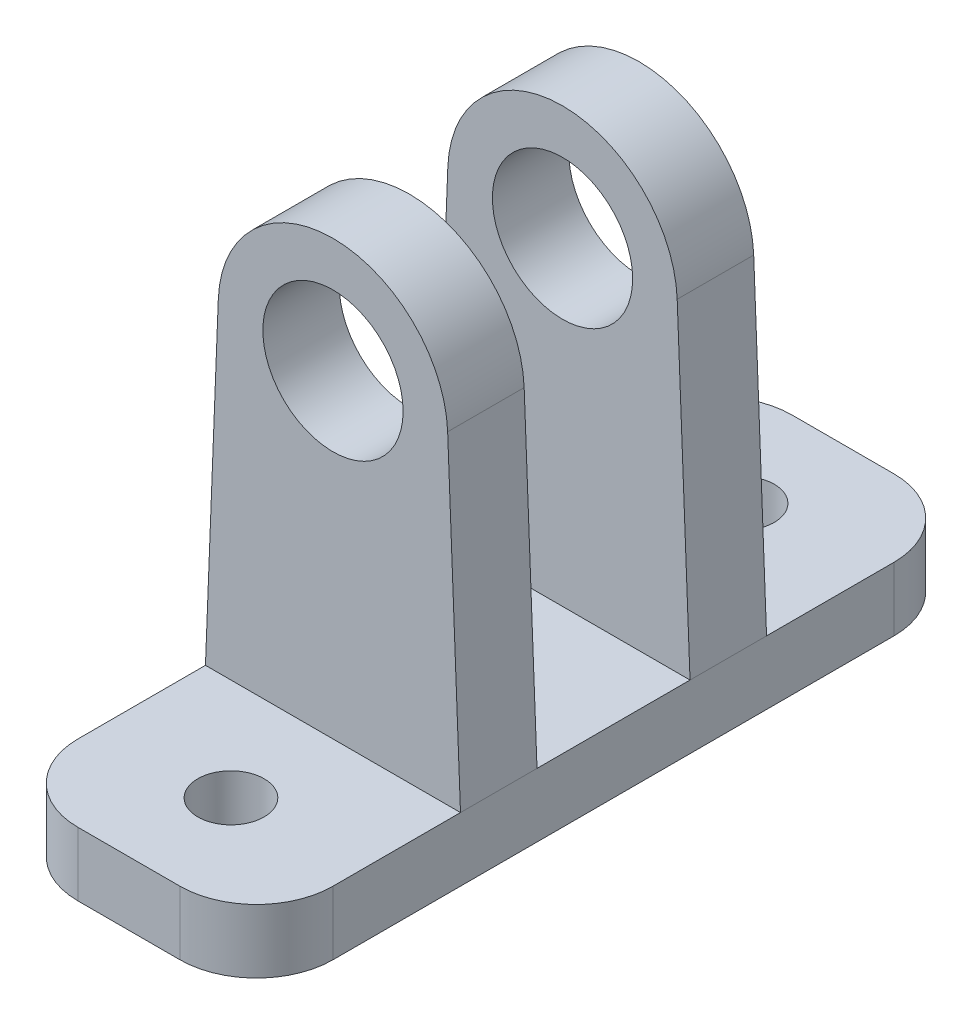
from build123d import *

# Parameters (mm, degrees)
SKETCH_1_W           = 100
SKETCH_1_H           = 120
BOSS_EXTRUDE_1_DEPTH = 25
SKETCH_2_R           = 27.5
BOSS_EXTRUDE_2_DEPTH = 30
SKETCH_4_W           = 15
SKETCH_4_H           = 25
BOSS_EXTRUDE_3_DEPTH = 10
SKETCH_5_W           = 100
SKETCH_5_H           = 280
SKETCH_5_R           = 13
BOSS_EXTRUDE_4_DEPTH = 25
FILLET_1_R           = 30


with BuildPart() as part:
    # Sketch 1 → Boss-Extrude 1 (new body)
    with BuildSketch(Plane(origin=(0, 0, 0), x_dir=(1, 0, 0), z_dir=(0, 1, 0))):
        Rectangle(SKETCH_1_W, SKETCH_1_H)
    extrude(amount=BOSS_EXTRUDE_1_DEPTH)

    # Sketch 2 → Boss-Extrude 2 (add)
    with BuildSketch(Plane.XY.offset(60)):
        with BuildLine():
            Line((-44.964550988, 151.785820395), (-50, 25))
            Line((-50, 25), (50, 25))
            Line((50, 25), (44.964550988, 151.785820395))
            ThreePointArc((44.964550988, 151.785820395), (0, 195), (-44.964550988, 151.785820395))
        make_face()
        with Locations((0, 150)):
            Circle(SKETCH_2_R, mode=Mode.SUBTRACT)
    boss_extrude_2 = extrude(amount=-BOSS_EXTRUDE_2_DEPTH)

    # Sketch 4 → Boss-Extrude 3 (add)
    with BuildSketch(Plane.XY.offset(60)):
        with Locations((0, 12.5)):
            Rectangle(SKETCH_4_W, SKETCH_4_H)
    boss_extrude_3 = extrude(amount=BOSS_EXTRUDE_3_DEPTH)

    # Mirror 1: Boss-Extrude 2, Boss-Extrude 3 across plane
    add(boss_extrude_2.mirror(Plane.XY))
    add(boss_extrude_3.mirror(Plane.XY))

    # Sketch 5 → Boss-Extrude 4 (add)
    with BuildSketch(Plane.XZ):
        Rectangle(SKETCH_5_W, SKETCH_5_H)
        with Locations(Location((0, -100, 0), (0, 0, 270))):
            Circle(SKETCH_5_R, mode=Mode.SUBTRACT)
        with Locations(Location((0, 100, 0), (0, 0, 270))):
            Circle(SKETCH_5_R, mode=Mode.SUBTRACT)
    extrude(amount=-BOSS_EXTRUDE_4_DEPTH)

    # Fillet 1
    fillet_1_edges = [part.edges().sort_by_distance(p)[0] for p in [
        (-50, 12.5, -140),
        (50, 12.5, 140),
        (50, 12.5, -140),
        (-50, 12.5, 140),
    ]]
    fillet(fillet_1_edges, radius=FILLET_1_R)


solid = part.part
